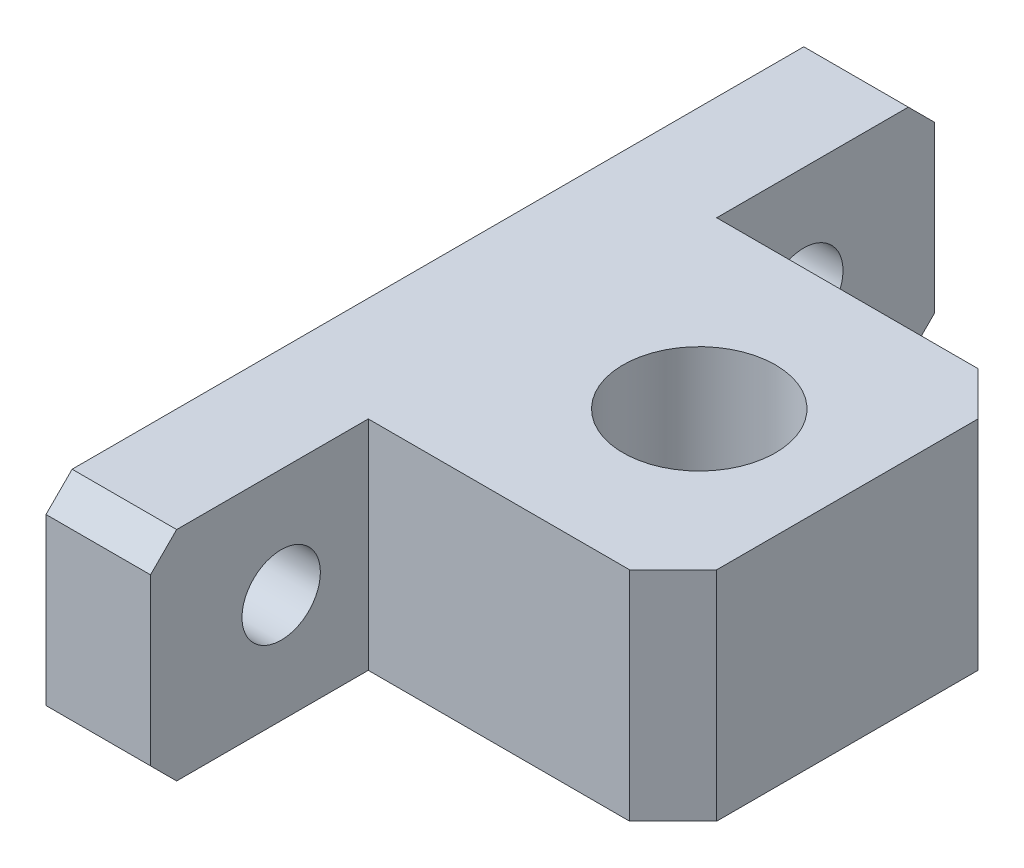
from build123d import *

# Parameters (mm, degrees)
SKETCH_1_W            = 90
SKETCH_1_H            = 25
EXTRUDE_1_DEPTH       = 12
SKETCH_2_W            = 40
SKETCH_2_H            = 25
EXTRUDE_2_DEPTH       = 35
HOLE_WIZARD_M20_1_D   = 17.5
HOLE_WIZARD_9_0_9_1_D = 9
CHAMFER_1_SIZE        = 5
CHAMFER_2_SIZE        = 3


with BuildPart() as part:
    # 草图1 → 凸台-拉伸1 (new body)
    with BuildSketch(Plane(origin=(0, 0, 0), x_dir=(0, 0, -1), z_dir=(1, 0, 0))):
        Rectangle(SKETCH_1_W, SKETCH_1_H)
    extrude(amount=EXTRUDE_1_DEPTH)

    # 草图2 → 凸台-拉伸2 (add)
    with BuildSketch(Plane(origin=(12, 0, 0), x_dir=(0, 0, -1), z_dir=(1, 0, 0))):
        Rectangle(SKETCH_2_W, SKETCH_2_H)
    extrude(amount=EXTRUDE_2_DEPTH)

    # M20 螺纹孔1 (through all)
    with Locations(Plane(origin=(0, -12.5, 0), x_dir=(-1, 0, 0), z_dir=(0, -1, 0))):
        with Locations((-30, 0)):
            Hole(HOLE_WIZARD_M20_1_D / 2)

    # Ø9.0 (9) 直径孔1 (through all)
    with Locations(Plane(origin=(12, 0, 0), x_dir=(0, 0, -1), z_dir=(1, 0, 0))):
        with Locations((-30, 0), (30, 0)):
            Hole(HOLE_WIZARD_9_0_9_1_D / 2)

    # 倒角1
    chamfer_1_edges = [part.edges().sort_by_distance(p)[0] for p in [
        (47, 0, -20),
        (47, 0, 20),
    ]]
    chamfer(chamfer_1_edges, length=CHAMFER_1_SIZE)

    # 倒角2
    chamfer_2_edges = [part.edges().sort_by_distance(p)[0] for p in [
        (6, -12.5, -45),
        (6, -12.5, 45),
        (6, 12.5, 45),
        (6, 12.5, -45),
    ]]
    chamfer(chamfer_2_edges, length=CHAMFER_2_SIZE)


solid = part.part
